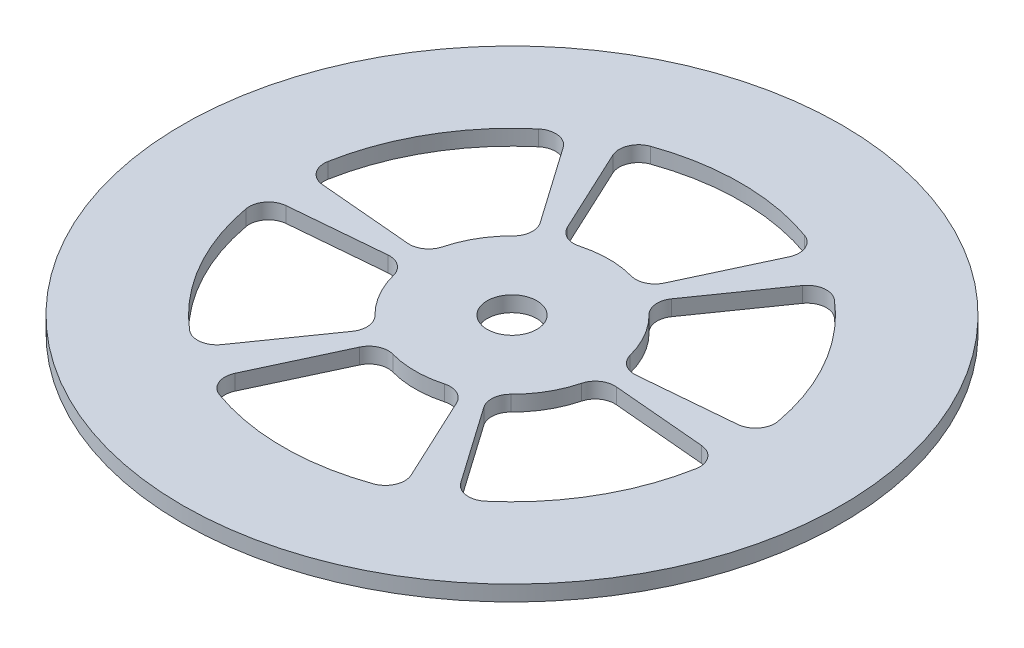
SolidWorks part; units mm, degrees
material "丙烯酸(中高冲击)"
ref_plane "Front Plane" through (0, 0, 0) normal (0, 0, 1) x (1, 0, 0)
ref_plane "Top Plane" through (0, 0, 0) normal (0, 1, 0) x (1, 0, 0)
ref_plane "Right Plane" through (0, 0, 0) normal (1, 0, 0) x (0, 0, -1)
other "Configuration Table"
sketch "Sketch1" plane through (0, 0, 0) normal (0, 1, 0) x (1, 0, 0)
  circle A0 centre (0, 0) radius 85
  circle A1 centre (0, 0) radius 6.4
  point P12 (-3.1161, 0.2799)
  point P16 (0, 0)
  dimension "D1" = 170
  dimension "D2" = 12.8
extrude "Boss-Extrude1" add sketch "Sketch1" along normal blind 4
sketch "Sketch2" plane through (0, 4, 0) normal (0, 1, 0) x (1, 0, 0)
  line L0 (10.5655, 22.6577) -> (24.9345, 53.4722)
  line L1 (0, 0) -> (0, 53.6207) construction
  line L2 (-10.5655, 22.6577) -> (-24.9345, 53.4722)
  line L3 (14.3394, 20.4788) -> (33.841, 48.33)
  line L4 (24.9049, 2.1789) -> (58.7755, 5.1422)
  line L5 (24.9049, -2.1789) -> (58.7755, -5.1422)
  line L6 (14.3394, -20.4788) -> (33.841, -48.33)
  line L7 (10.5655, -22.6577) -> (24.9345, -53.4722)
  line L8 (-10.5655, -22.6577) -> (-24.9345, -53.4722)
  line L9 (-14.3394, -20.4788) -> (-33.841, -48.33)
  line L10 (-24.9049, -2.1789) -> (-58.7755, -5.1422)
  line L11 (-24.9049, 2.1789) -> (-58.7755, 5.1422)
  line L12 (-14.3394, 20.4788) -> (-33.841, 48.33)
  arc A5 (10.5655, 22.6577) -> (-10.5655, 22.6577) centre (0, 0) ccw
  arc A6 (24.9345, 53.4722) -> (-24.9345, 53.4722) centre (0, 0) ccw
  arc A7 (24.9049, 2.1789) -> (14.3394, 20.4788) centre (0, 0) ccw
  arc A8 (58.7755, 5.1422) -> (33.841, 48.33) centre (0, 0) ccw
  arc A9 (14.3394, -20.4788) -> (24.9049, -2.1789) centre (0, 0) ccw
  arc A10 (33.841, -48.33) -> (58.7755, -5.1422) centre (0, 0) ccw
  arc A11 (-10.5655, -22.6577) -> (10.5655, -22.6577) centre (0, 0) ccw
  arc A12 (-24.9345, -53.4722) -> (24.9345, -53.4722) centre (0, 0) ccw
  arc A13 (-24.9049, -2.1789) -> (-14.3394, -20.4788) centre (0, 0) ccw
  arc A14 (-58.7755, -5.1422) -> (-33.841, -48.33) centre (0, 0) ccw
  arc A15 (-14.3394, 20.4788) -> (-24.9049, 2.1789) centre (0, 0) ccw
  arc A16 (-33.841, 48.33) -> (-58.7755, 5.1422) centre (0, 0) ccw
  point P13 (0, 0)
  point P30 (0, 0)
  dimension "D1" = 50
  dimension "D2" = 118
  dimension "D3" = 25
  dimension "D4" = 6
extrude "Cut-Extrude1" cut sketch "Sketch2" against normal blind 10
fillet "Fillet1" radius 5 24 edges at (10.5655, 2, -22.6577) (-10.5655, 2, -22.6577) (-14.3394, 2, -20.4788) (-24.9049, 2, -2.1789) (-24.9049, 2, 2.1789) (-10.5655, 2, 22.6577) (10.5655, 2, 22.6577) (14.3394, 2, 20.4788) (24.9049, 2, 2.1789) (24.9049, 2, -2.1789) (14.3394, 2, -20.4788) (-14.3394, 2, 20.4788) (-24.9345, 2, 53.4722) (-33.841, 2, 48.33) (-58.7755, 2, 5.1422) (-58.7755, 2, -5.1422) (-33.841, 2, -48.33) (-24.9345, 2, -53.4722) (24.9345, 2, 53.4722) (33.841, 2, 48.33) (58.7755, 2, 5.1422) (58.7755, 2, -5.1422) (33.841, 2, -48.33) (24.9345, 2, -53.4722)
